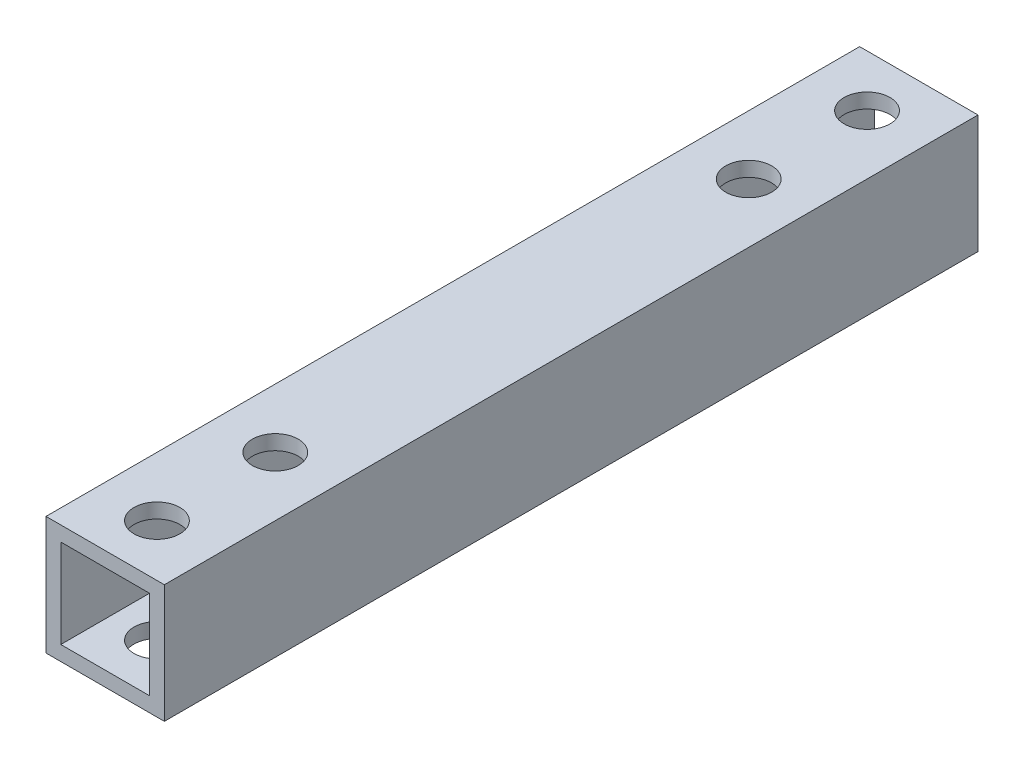
SolidWorks part; units mm, degrees
material "Thornel Mat VMA"
ref_plane "前视基准面" through (0, 0, 0) normal (0, 0, 1) x (1, 0, 0)
ref_plane "上视基准面" through (0, 0, 0) normal (0, 1, 0) x (1, 0, 0)
ref_plane "右视基准面" through (0, 0, 0) normal (1, 0, 0) x (0, 0, -1)
other "Configuration Table"
sketch "草图1" plane through (0, 0, 0) normal (0, 0, 1) x (1, 0, 0)
  line L0 (-3, 3) -> (3, 3)
  line L1 (-4, 4) -> (4, 4)
  line L2 (-4, 4) -> (-4, -4)
  line L3 (-4, -4) -> (4, -4)
  line L4 (4, 4) -> (4, -4)
  line L5 (-4, 4) -> (4, -4) construction
  line L6 (-4, -4) -> (4, 4) construction
  line L7 (3, 3) -> (3, -3)
  line L8 (-3, -3) -> (3, -3)
  line L9 (-3, 3) -> (-3, -3)
  point P0 (0, 0)
  dimension "D1" = 8
  dimension "D2" = 1
extrude "凸台-拉伸1" add sketch "草图1" against normal blind 55
sketch "草图3" plane through (0, 4, 0) normal (0, 1, 0) x (1, 0, 0)
  line L0 (0, 0) -> (0, 65.3909) construction
  line L1 (4, 0) -> (-4, 0) construction
  line L2 (4, 55) -> (-4, 55) construction
  circle A0 centre (0, 3.5) radius 1.55
  circle A1 centre (0, 11.5) radius 1.55
  circle A2 centre (0, 43.5) radius 1.55
  circle A3 centre (0, 51.5) radius 1.55
  dimension "D1" = 3.1
  dimension "D2" = 3.5
  dimension "D3" = 8
  dimension "D4" = 3.5
  dimension "D5" = 8
extrude "切除-拉伸1" cut sketch "草图3" against normal blind 55
